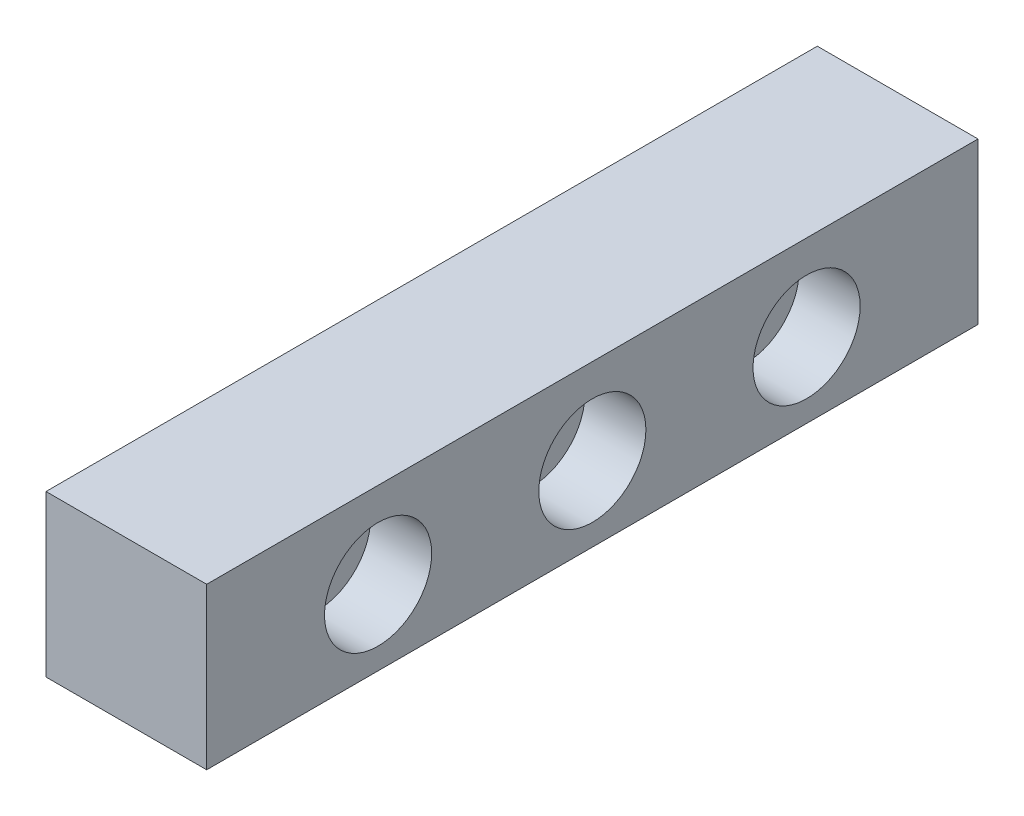
from build123d import *

# Parameters (mm, degrees)
SKETCH_1_W                = 72
SKETCH_1_H                = 15
EXTRUDE_1_DEPTH           = 15
HOLE_WIZARD_2_D           = 5.5
HOLE_WIZARD_2_CBORE_D     = 10
HOLE_WIZARD_2_CBORE_DEPTH = 5.7


with BuildPart() as part:
    # 草图1 → 凸台-拉伸1 (new body)
    with BuildSketch(Plane(origin=(0, 0, 0), x_dir=(0, 0, -1), z_dir=(1, 0, 0))):
        Rectangle(SKETCH_1_W, SKETCH_1_H)
    extrude(amount=EXTRUDE_1_DEPTH)

    # 打孔尺寸(%根据)内六角圆柱头螺钉的类型2 (through all)
    with Locations(Plane(origin=(15, 0, 0), x_dir=(0, 0, -1), z_dir=(1, 0, 0))):
        with Locations((-20, -0.5), (0, -0.5), (20, -0.5)):
            CounterBoreHole(HOLE_WIZARD_2_D / 2, HOLE_WIZARD_2_CBORE_D / 2, HOLE_WIZARD_2_CBORE_DEPTH)


solid = part.part
